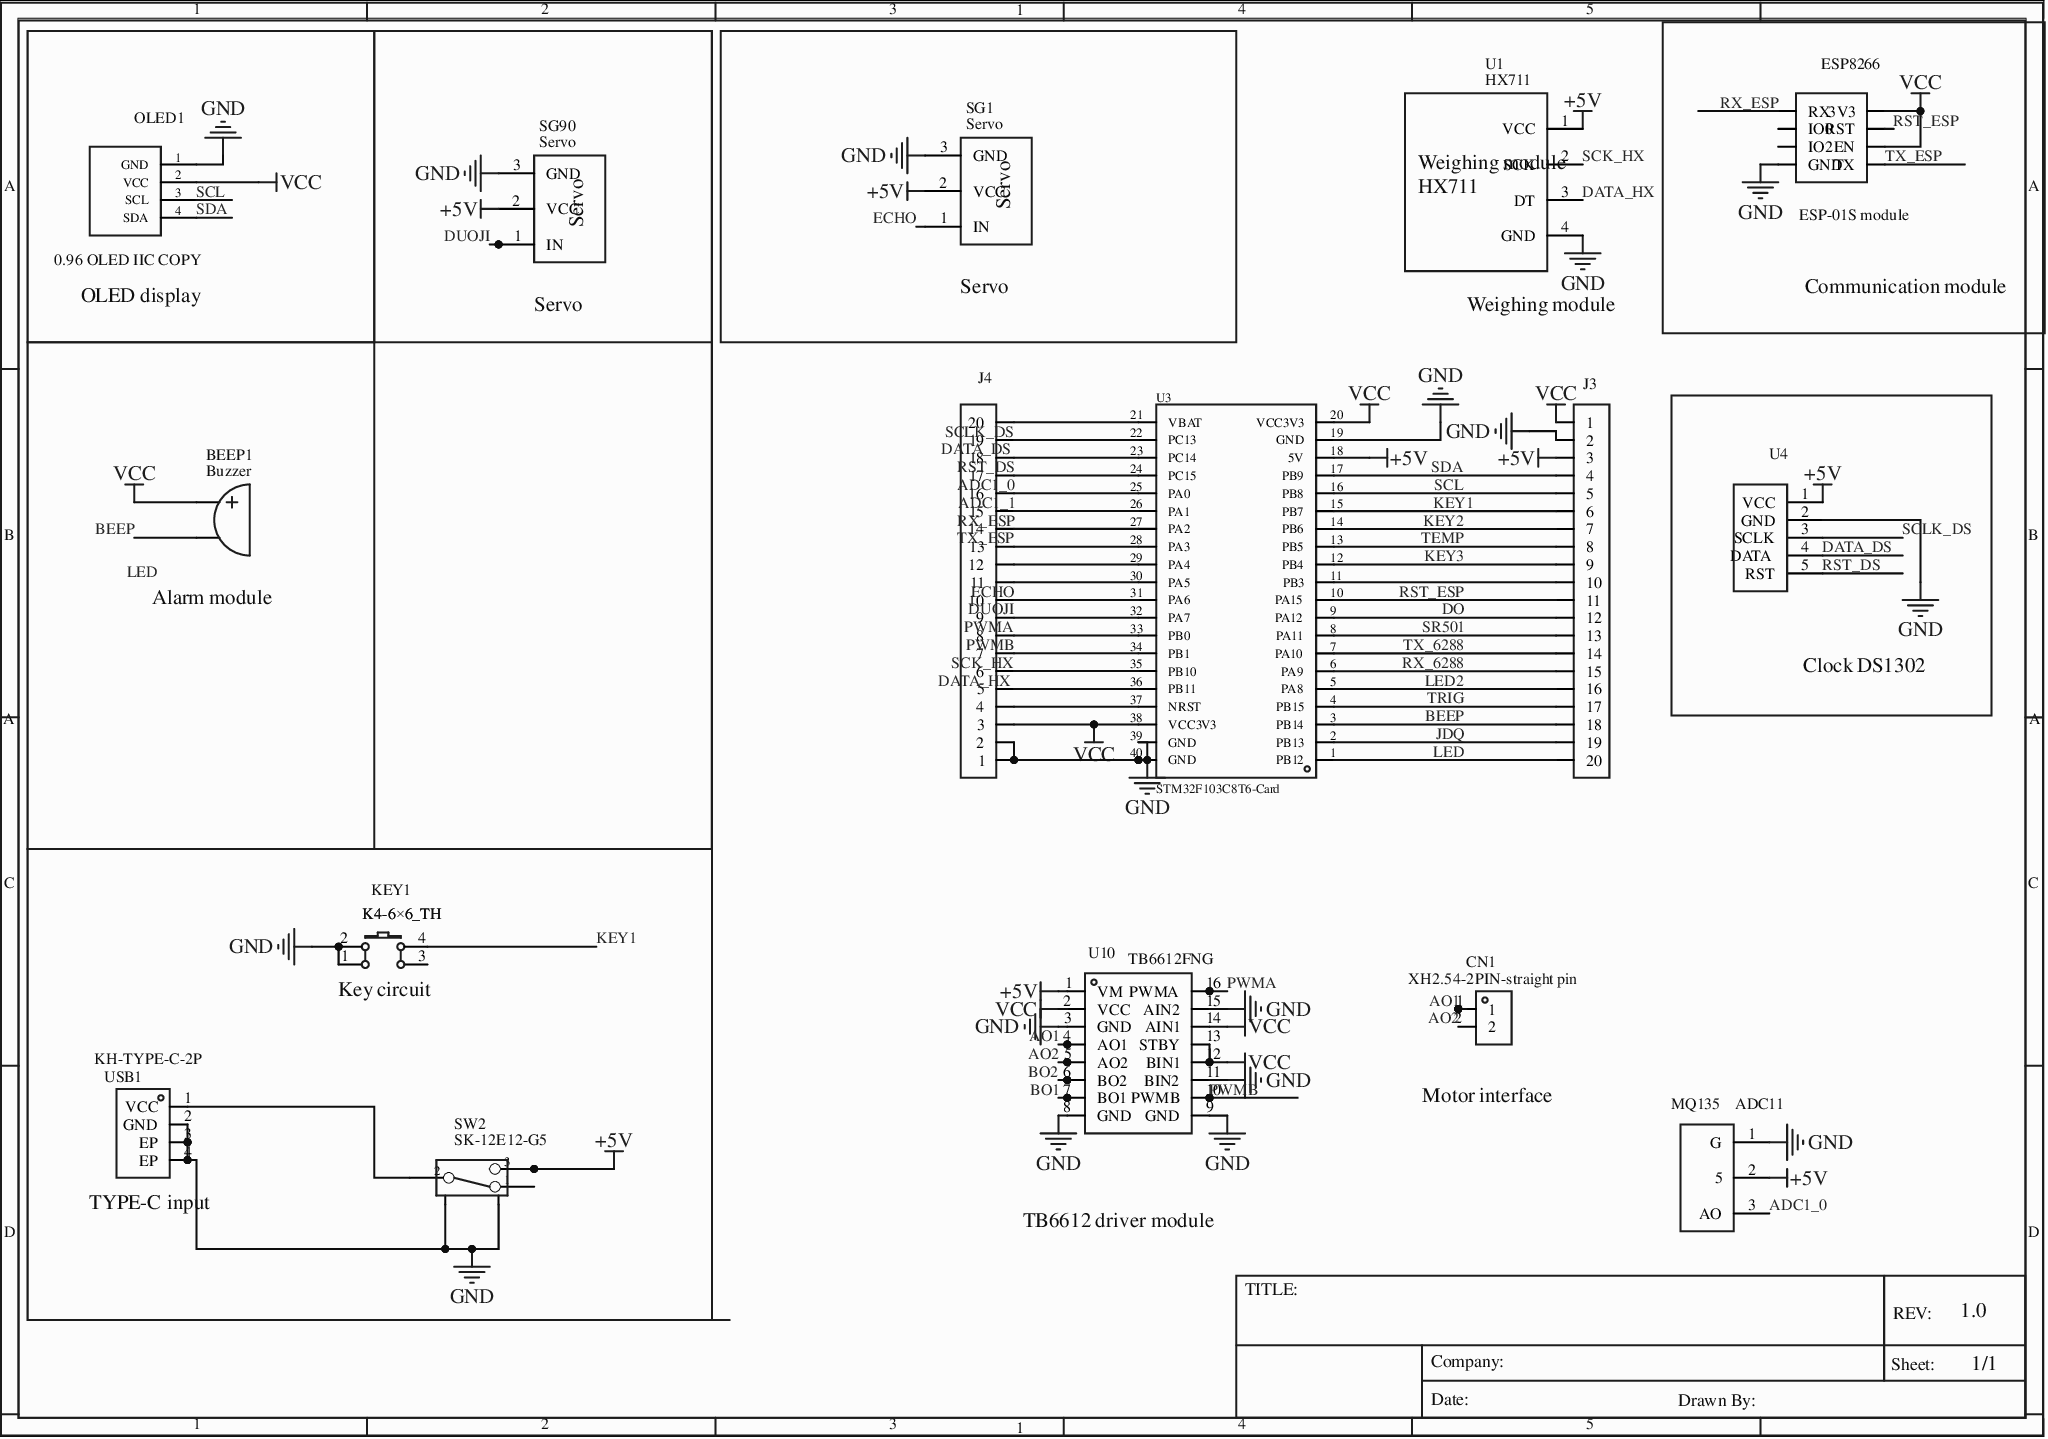
[diagram p0: MISC49936-3.schdoc]
# Altium project MISC49936-2.PrjPcb
1 sheet, 16 parts. Net scope: global (net labels, ports and power ports of the same name join across sheets).
Board file: MISC49936.pcbdoc

## Sheet MISC49936-3.schdoc
size 292 x 205 mm; Name: MISC49936; @Project Name: MISC49936; REV: 1.0; Sheet: 1/1; Manufacturer Part: ?

### Parts
ADC11  MQ135  [HDR-TH_3P-P2.54-V-F]
BEEP1  Buzzer  [BUZ-TH_BD11.8-P7.60_XHXDZ-TMB12065]
CN1  XH2.54-2PIN-straight pin  [CONN-TH_XH2.54-2P]
ESP8266  ESP-01S module  [WIFIM-TH_ESP-01S]
J3  HDR-M-2.54_1x20  [HDR-M-2.54_1X20]  (value not drawn)
J4  HDR-M-2.54_1x20  [HDR-M-2.54_1X20]  (value not drawn)
KEY1  K4-6×6_TH  [KEY-TH_4P-L6.0-W6.0-P4.50-LS6.5]
OLED1  0.96 OLED IIC COPY  [OLED-TH_4P-L23.44-W19.0_ER-OLEDM0.66-1W-I2C]
SG1  Servo  [HDR-TH_3P-P2.54-V-F]
SG90  Servo  [HDR-TH_3P-P2.54-V-F]
SW2  SK-12E12-G5  [SW-TH_SK-12E12-G5]
U1  HX711  [HDR-TH_4P-P2.54-V-F]
U3  STM32F103C8T6-Card  [CONN-TH_L53.3-W22.9_STM32F103C8T6-CARD]
U4  Clock DS1302  [HDR-TH_5P-P2.54-V-F]
U10  TB6612FNG  [tb6612]
USB1  KH-TYPE-C-2P  [USB-SMD_KH-TYPE-C-2P]

### Blocks framed on the sheet
OLED display: OLED1
Servo: SG90
Servo: SG1
Communication module: ESP8266
Alarm module: BEEP1

### Nets
+5V: ADC11.2(5) J3.3 SG1.2(VCC) SG90.2(VCC) SW2.3 U1.1(VCC) U3.18(5V) U4.1(VCC) U10.1(VM)
GND: ADC11.1(G) ESP8266.5(GND) J3.2 J4.1 J4.2 KEY1.1 KEY1.2 OLED1.1(GND) SG1.3(GND) SG90.3(GND) SW2.4 SW2.5 U1.4(GND) U3.19(GND) U3.39(GND) U3.40(GND) U4.2(GND) U10.3(GND) U10.8(GND) U10.9(GND) U10.11(BIN2) U10.15(AIN2) USB1.2(GND) USB1.3(EP) USB1.4(EP)
VCC: BEEP1.1(A) ESP8266.1(3V3) ESP8266.3(EN) J3.1 J4.3 OLED1.2(VCC) U3.20(VCC3V3) U3.38(VCC3V3) U10.2(VCC) U10.12(BIN1) U10.13(STBY) U10.14(AIN1)
ADC1_0: ADC11.3(AO) J4.16 U3.25(PA0)
ADC1_1: J4.15 U3.26(PA1)
AO1: CN1.1 U10.4(AO1)
AO2: CN1.2 U10.5(AO2)
BEEP: BEEP1.2(B) J3.18 U3.3(PB14)
BO1: U10.7(BO1)
BO2: U10.6(BO2)
DATA_DS: J4.18 U3.23(PC14) U4.4(DATA)
DATA_HX: J4.5 U1.3(DT) U3.36(PB11)
DO: J3.12 U3.9(PA12)
DUOJI: J4.9 SG90.1(IN) U3.32(PA7)
ECHO: J4.10 SG1.1(IN) U3.31(PA6)
JDQ: J3.19 U3.2(PB13)
KEY1: J3.6 KEY1.4 U3.15(PB7)
KEY2: J3.7 U3.14(PB6)
KEY3: J3.9 U3.12(PB4)
LED: J3.20 U3.1(PB12)
LED2: J3.16 U3.5(PA8)
PWMA: J4.8 U3.33(PB0) U10.16(PWMA)
PWMB: J4.7 U3.34(PB1) U10.10(PWMB)
RST_DS: J4.17 U3.24(PC15) U4.5(RST)
RST_ESP: ESP8266.2(RST) J3.11 U3.10(PA15)
RX_6288: J3.15 U3.6(PA9)
RX_ESP: ESP8266.8(RX) J4.14 U3.27(PA2)
SCK_HX: J4.6 U1.2(SCK) U3.35(PB10)
SCL: J3.5 OLED1.3(SCL) U3.16(PB8)
SCLK_DS: J4.19 U3.22(PC13) U4.3(SCLK)
SDA: J3.4 OLED1.4(SDA) U3.17(PB9)
SR501: J3.13 U3.8(PA11)
TEMP: J3.8 U3.13(PB5)
TRIG: J3.17 U3.4(PB15)
TX_6288: J3.14 U3.7(PA10)
TX_ESP: ESP8266.4(TX) J4.13 U3.28(PA3)
NetJ3_10: J3.10 U3.11(PB3)
NetJ4_4: J4.4 U3.37(NRST)
NetJ4_11: J4.11 U3.30(PA5)
NetJ4_12: J4.12 U3.29(PA4)
NetJ4_20: J4.20 U3.21(VBAT)
NetSW2_2: SW2.2 USB1.1(VCC)

Not connected (* = marked no-connect by the designer): ESP8266 6(IO2)* 7(IO0)*; KEY1 3*; SW2 1*

### Notes on the sheet
- (near U1) Weighing module
- (near KEY1) K4-6×6_TH
- (near KEY1) Key circuit
- (near CN1) Motor interface
- (near USB1) TYPE-C input
- TB6612 driver module
- Labels drawn without touching a wire or pin: LED
- 1
- 2
- 3
- 4
- 5
- A
- B
- C
- D
- TITLE:
- Company:
- Sheet:
- REV:
- 1.0
- 1/1
- Date:
- Drawn By:

### Library data of the parts
ADC11 = MQ135: Convert to PCB: yes; Origin Footprint: Water level/TDS; UniqueId: gge2642c5a8ee4a941d; Device: MQ135; Add into BOM: yes; SymbolName: MQ135
BEEP1 = 蜂鸣器: Convert to PCB: yes; Origin Footprint: Active buzzer; UniqueId: ggeb413ea6f478d18df; Device: Buzzer; Add into BOM: yes; SymbolName: Buzzer
CN1 = XH2.54-2PIN-直针: Manufacturer: null; Convert to PCB: yes; UniqueId: gge8ec7bbd982bc0e91; ModelId: dc9654a6caad4c20aab3bc231ea458cf; Device: XH2.54-2PIN-straight pin; Supplier: LCSC; Supplier Part: C9900011425; Manufacturer Part: XH2.54-2PIN-直针; JLCPCB Part Class: Extended Part; Add into BOM: yes; SymbolName: XH2.54-2PIN-straight pin; FootprintName: CONN-TH_XH2.54-2P; ModelName: CONN-TH_XH2.54-2P
ESP8266 = ESP-01S模块: Convert to PCB: yes; Origin Footprint: ESP01S; UniqueId: ggefc7376b53e6a6a91; Device: ESP-01S module; Add into BOM: yes; SymbolName: ESP-01S module
J3 = HDR-M-2.54_1x20: Convert to PCB: yes; ModelId: 3a23733f0ee3481e9756e4311e8a6823; Device: HDR-M-2.54_1x20; Supplier Part: C50981; Supplier: LCSC; Add into BOM: yes; Symbol: HDR-M-2.54_1x20; FootprintName: HDR-M-2.54_1X20; ModelName: HDR-M-2.54_1x20
J4 = HDR-M-2.54_1x20: Convert to PCB: yes; UniqueId: ggebe34872adfe08dcf; ModelId: 3a23733f0ee3481e9756e4311e8a6823; Device: HDR-M-2.54_1x20; Supplier Part: C50981; Supplier: LCSC; Add into BOM: yes; SymbolName: HDR-M-2.54_1x20; FootprintName: HDR-M-2.54_1X20; ModelName: HDR-M-2.54_1x20
KEY1 = K2-1102DP-E4SW-04: Manufacturer: 韩国韩荣; Convert to PCB: yes; UniqueId: ggeb62aab1eaed42ba1; ModelId: 84a564898aee4f89a3c7a00b1a1f425b; Device: K2-1102DP-E4SW-04; Supplier: LCSC; Supplier Part: C136684; Manufacturer Part: K2-1102DP-E4SW-04; Add into BOM: yes; SymbolName: K4-6×6_TH; FootprintName: KEY-TH_4P-L6.0-W6.0-P4.50-LS6.5; ModelName: KEY-TH_4P-L6.0-W6.0-P4.50-LS6.5
OLED1 = 0.96 OLED IIC COPY: Convert to PCB: yes; Origin Footprint: OLED-TH_OLED0.96-IIC; UniqueId: gge9c5712e397c8a31c; Device: 0.96 OLED IIC COPY; Add into BOM: yes; SymbolName: 0.96 OLED IIC COPY
SG1 = 舵机: Convert to PCB: yes; Origin Footprint: SG90; UniqueId: ggee092c517e5406696; Device: Servo; Add into BOM: yes; SymbolName: Servo
SG90 = 舵机: Convert to PCB: yes; Origin Footprint: SG90; UniqueId: gge84acc697b53da6f4; Device: Servo; Add into BOM: yes; SymbolName: Servo
SW2 = SK-12E12-G5: Manufacturer: Rectangular Connectors - Contacts; Convert to PCB: yes; UniqueId: ggeb928d096a38884b7; ModelId: 63ecb7c3b60e41c79481f203e3e77e6b; Device: SK-12E12-G5; Supplier: LCSC; Supplier Part: C136720; Manufacturer Part: SK-12E12-G5; Add into BOM: yes; SymbolName: SK-12E12-G5; FootprintName: SW-TH_SK-12E12-G5; ModelName: SW-TH_SK-12E12-G5
U1 = HX711: Convert to PCB: yes; UniqueId: gge8f0da4cc9a27c4bc; Device: HX711; Add into BOM: yes; Origin Footprint: HX711; SymbolName: HX711
U3 = STM32F103C8T6-Card: AddInBom: yes; ModelId: 70cdd142a616427fa7f75b03dcb285590819f05c4eef4c71ace90d822a990e87; ModelTransform: 2310.042,898.9982,0,0,0,0,90.551,0,-236.22; Symbol: STM32F103C8T6-CARD; Device: STM32F103C8T6-Card; LCSC Part Name: STM32F103C8T6-Card; SupplierPart: C9900077949; ManufacturerPart: STM32F103C8T6-Card; Supplier Footprint: 插件; JLCPCB Part Class: Extended Part; Supplier: LCSC; ConvertToPcb: yes; FootprintName: CONN-TH_L53.3-W22.9_STM32F103C8T6-CARD; ModelName: CONN-TH_L53.3-W22.9_STM32F103C8T6-CARD
U4 = 时钟DS1302: Convert to PCB: yes; Origin Footprint: DS1302 module; UniqueId: gge04ee39644e7919d9; Device: Clock DS1302; Add into BOM: yes; SymbolName: Clock DS1302
U10 = TB6612FNG: Convert to PCB: yes; UniqueId: gge87489b2c6750c2e3; Device: TB6612FNG; Add into BOM: yes; Origin Footprint: TB6612FNG; SymbolName: TB6612FNG
USB1 = KH-TYPE-C-2P: Manufacturer: kinghelm(金航标); Convert to PCB: yes; UniqueId: gge9c60ea97b35b58cd; ModelId: 4464b34a7d0f48c2b8c2350e914c93f5; Device: KH-TYPE-C-2P; Supplier: LCSC; Supplier Part: C2919656; Manufacturer Part: KH-TYPE-C-2P; JLCPCB Part Class: Extended Part; Add into BOM: yes; SymbolName: KH-TYPE-C-2P; FootprintName: USB-SMD_KH-TYPE-C-2P; ModelName: USB-SMD_KH-TYPE-C-2P